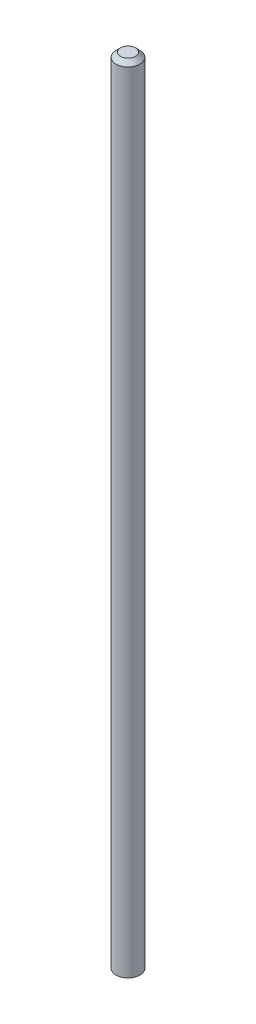
from build123d import *

# Parameters (mm, degrees)
SKETCH1_R           = 8
BOSS_EXTRUDE1_DEPTH = 531.5
CHAMFER1_SIZE       = 3


with BuildPart() as part:
    # Sketch1 → Boss-Extrude1 (new body)
    with BuildSketch(Plane(origin=(0, 0, 0), x_dir=(1, 0, 0), z_dir=(0, 1, 0))):
        with Locations(Location((0, 0, 0), (0, 0, 270))):
            Circle(SKETCH1_R)
    extrude(amount=BOSS_EXTRUDE1_DEPTH)

    # Chamfer1
    chamfer1_edges = [part.edges().sort_by_distance(p)[0] for p in [
        (0, 531.5, -8),
    ]]
    chamfer(chamfer1_edges, length=CHAMFER1_SIZE)


solid = part.part
